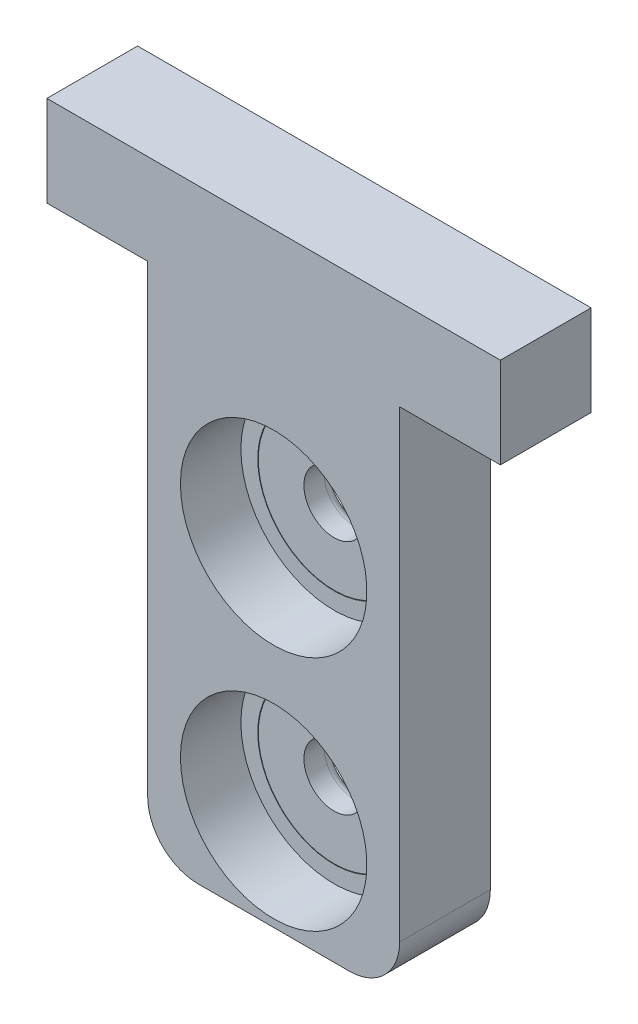
from build123d import *

# Parameters (mm, degrees)
SKETCH_1_W             = 50
SKETCH_1_H             = 120
EXTRUDE_1_DEPTH        = 18
SKETCH_2_W             = 90
SKETCH_2_H             = 18
EXTRUDE_2_DEPTH        = 18
FILLET_1_R             = 10
SKETCH_3_R             = 6
CUT_EXTRUDE_1_DEPTH    = 78.129760793
SKETCH_4_R             = 15.150210707
SKETCH_4_R_2           = 15.050210707
CUT_EXTRUDE_2_DEPTH    = 78.129760793
PATTERN_LINEAR_1_COUNT = 2
PATTERN_LINEAR_1_PITCH = 47
FILLET_2_R             = 2
FILLET_3_R             = 2
SKETCH_5_R             = 18.5
CUT_EXTRUDE_3_DEPTH    = 12


with BuildPart() as part:
    # 草图1 → 凸台-拉伸1 (new body)
    with BuildSketch(Plane.XY):
        Rectangle(SKETCH_1_W, SKETCH_1_H)
    extrude(amount=EXTRUDE_1_DEPTH)

    # 草图2 → 凸台-拉伸2 (add)
    with BuildSketch(Plane(origin=(0, 60, 0), x_dir=(1, 0, 0), z_dir=(0, 1, 0))):
        with Locations((0, -9)):
            Rectangle(SKETCH_2_W, SKETCH_2_H)
    extrude(amount=-EXTRUDE_2_DEPTH)

    # 圆角1
    fillet_1_edges = [part.edges().sort_by_distance(p)[0] for p in [
        (25, -60, 9),
        (-25, -60, 9),
    ]]
    fillet(fillet_1_edges, radius=FILLET_1_R)

    # 草图3 → 切除-拉伸1 (cut, through all)
    with BuildSketch(Plane(origin=(0, 0, 0), x_dir=(-1, 0, 0), z_dir=(0, 0, -1))):
        with Locations((0, -40)):
            Circle(SKETCH_3_R)
    cut_extrude_1 = extrude(amount=-CUT_EXTRUDE_1_DEPTH, mode=Mode.SUBTRACT)

    # 草图4 → 切除-拉伸2 (cut, through all)
    with BuildSketch(Plane(origin=(0, 0, 0), x_dir=(-1, 0, 0), z_dir=(0, 0, -1))):
        with Locations((0, -40)):
            Circle(SKETCH_4_R)
        with Locations((0, -40)):
            Circle(SKETCH_4_R_2, mode=Mode.SUBTRACT)
    cut_extrude_2 = extrude(amount=-CUT_EXTRUDE_2_DEPTH, mode=Mode.SUBTRACT)


with BuildPart() as cut_extrude_2_piece_1:
    # of the separate pieces the step leaves, piece 1, a body of its own (cut_extrude_2_pieces)
    add(part.part.solids().sort_by_distance((-25, -50, 0))[0])

    # 阵列(线性)1: 切除-拉伸1, 切除-拉伸2 ×2
    with Locations(*[(0, i * PATTERN_LINEAR_1_PITCH, 0) for i in range(1, PATTERN_LINEAR_1_COUNT)]):
        add(cut_extrude_1, mode=Mode.SUBTRACT)
        add(cut_extrude_2, mode=Mode.SUBTRACT)

    # 圆角3
    fillet_3_edges = [cut_extrude_2_piece_1.edges().sort_by_distance(p)[0] for p in [
        (6, 7, 18),
        (6, 7, 0),
        (15.050210707, 7, 18),
        (15.050210707, 7, 0),
    ]]
    fillet(fillet_3_edges, radius=FILLET_3_R)


with BuildPart() as cut_extrude_2_piece_2:
    # of the separate pieces the step leaves, piece 2, a body of its own (cut_extrude_2_pieces)
    add(part.part.solids().sort_by_distance((-15.050210707, -40, 0))[0])

    # 圆角2
    fillet_2_edges = [cut_extrude_2_piece_2.edges().sort_by_distance(p)[0] for p in [
        (6, -40, 18),
        (6, -40, 0),
        (15.050210707, -40, 18),
        (15.050210707, -40, 0),
    ]]
    fillet(fillet_2_edges, radius=FILLET_2_R)


with BuildPart() as cut_extrude_3_tool:
    # 草图5 → 切除-拉伸3 (new body)
    with BuildSketch(Plane(origin=(0, 0, 18), x_dir=(-1, 0, 0), z_dir=(0, 0, -1))):
        with Locations((0, -40)):
            Circle(SKETCH_5_R)
        with Locations((0, 7)):
            Circle(SKETCH_5_R)
    extrude(amount=CUT_EXTRUDE_3_DEPTH)


with BuildPart() as cut_extrude_2_piece_1_1:
    add(cut_extrude_2_piece_1.part)

    # 切除-拉伸3: cut by cut_extrude_3_tool
    add(cut_extrude_3_tool.part, mode=Mode.SUBTRACT)


with BuildPart() as cut_extrude_2_piece_2_1:
    add(cut_extrude_2_piece_2.part)

    # 切除-拉伸3: cut by cut_extrude_3_tool
    add(cut_extrude_3_tool.part, mode=Mode.SUBTRACT)


solid = Compound([cut_extrude_2_piece_1_1.part, cut_extrude_2_piece_2_1.part])
